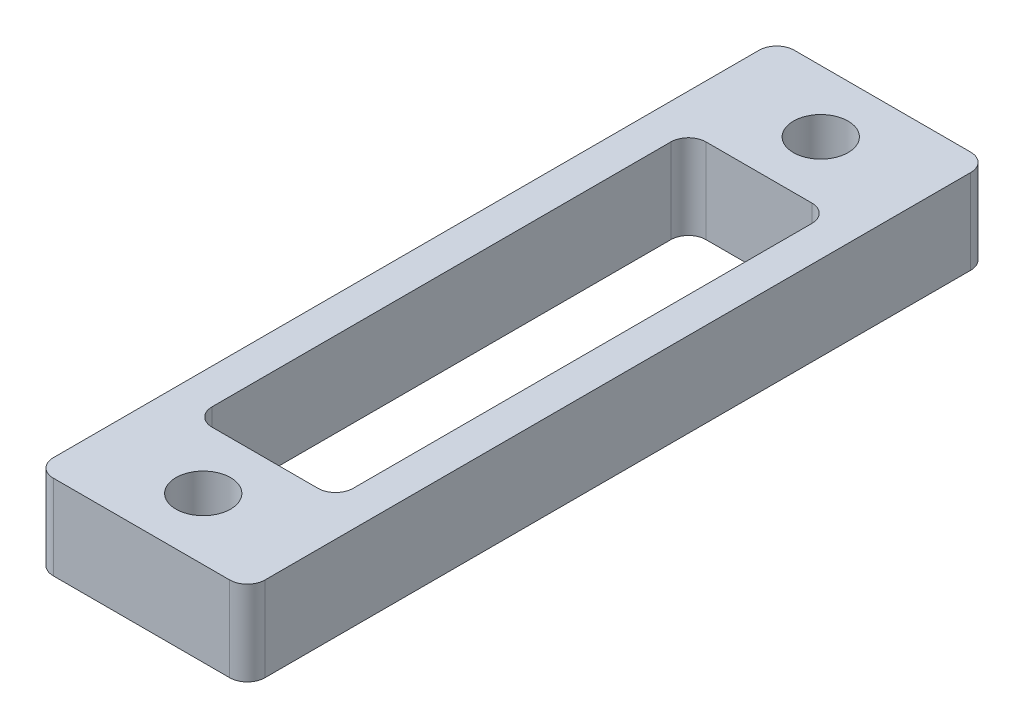
SolidWorks part; units mm, degrees
material "尼龙 101"
ref_plane "前视基准面" through (0, 0, 0) normal (0, 0, 1) x (1, 0, 0)
ref_plane "上视基准面" through (0, 0, 0) normal (0, 1, 0) x (1, 0, 0)
ref_plane "右视基准面" through (0, 0, 0) normal (1, 0, 0) x (0, 0, -1)
other "Configuration Table"
sketch "草图1" plane through (0, 0, 0) normal (0, 1, 0) x (1, 0, 0)
  line L0 (-6, 38.5) -> (6, 38.5)
  line L1 (-6, 3.5) -> (6, 3.5)
  line L2 (-6, 3.5) -> (-6, -3.5)
  line L3 (-6, -3.5) -> (6, -3.5)
  line L4 (6, 3.5) -> (6, -3.5)
  line L5 (-6, 3.5) -> (6, -3.5) construction
  line L6 (-6, -3.5) -> (6, 3.5) construction
  line L7 (-6, 38.5) -> (-6, 31.5)
  line L8 (-6, 31.5) -> (6, 31.5)
  line L9 (6, 38.5) -> (6, 31.5)
  line L10 (-6, 38.5) -> (6, 31.5) construction
  line L11 (-6, 31.5) -> (6, 38.5) construction
  line L12 (-6, 31.5) -> (-6, 3.5)
  line L13 (6, 31.5) -> (6, 3.5)
  line L14 (-4, 31.5) -> (-4, 3.5)
  line L15 (4, 31.5) -> (4, 3.5)
  circle A0 centre (0, 0) radius 1.55
  circle A1 centre (0, 35) radius 1.55
  dimension "D1" = 3.1
  dimension "D5" = 35
  dimension "D2" = 12
  dimension "D3" = 7
  dimension "D6" = 2
  dimension "D7" = 2
  dimension "D4" = 2
extrude "凸台-拉伸1" add sketch "草图1" along normal blind 4.8 contours L14 L8 L12 L1 | L9 L0 L7 L8 A1 | L8 L15 L1 L13 | L4 L1 L2 L3 A0
fillet "圆角1" radius 1 8 edges at (6, 2.4, 3.5) (-6, 2.4, 3.5) (-4, 2.4, -3.5) (4, 2.4, -3.5) (4, 2.4, -31.5) (-6, 2.4, -38.5) (6, 2.4, -38.5) (-4, 2.4, -31.5)
